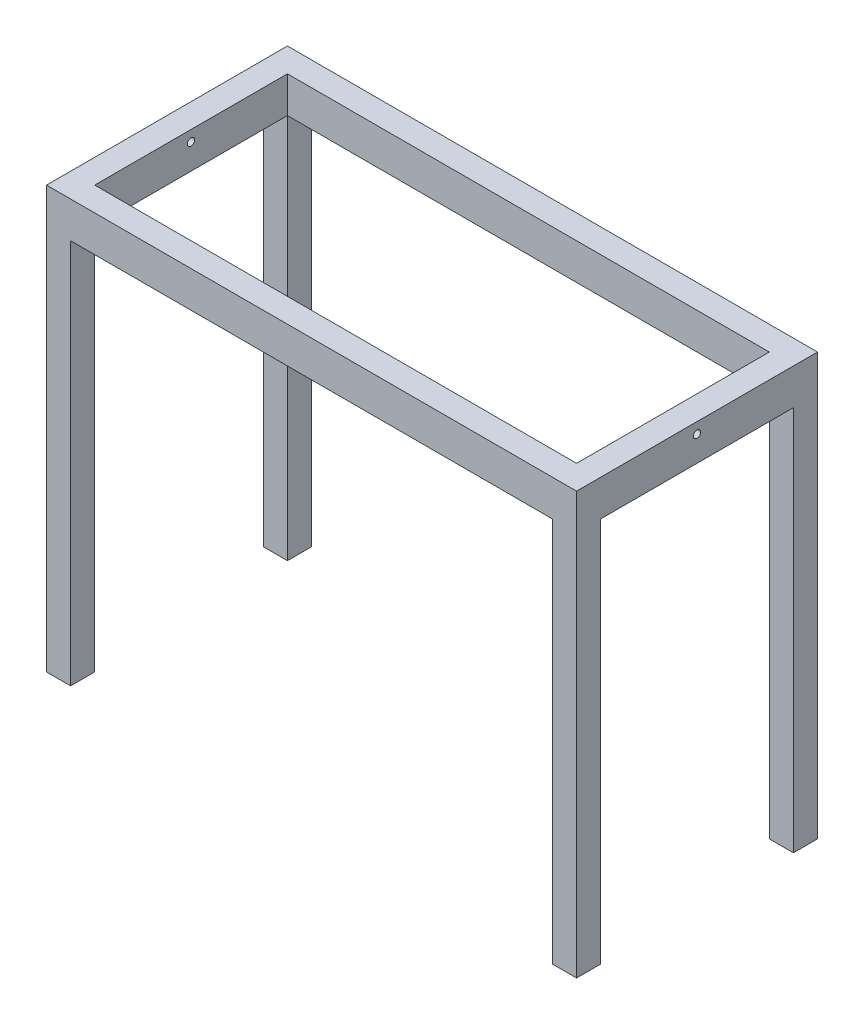
from build123d import *

# Parameters (mm, degrees)
SKETCH1_W               = 1100
SKETCH1_H               = 500
SKETCH1_W_2             = 1000
SKETCH1_H_2             = 400
BOSS_EXTRUDE1_DEPTH     = 75
SKETCH2_W               = 50
SKETCH2_H               = 50
BOSS_EXTRUDE2_DEPTH     = 800
CUT_EXTRUDE1_DEPTH      = 1383.931668594
CUT_EXTRUDE1_DEPTH_BACK = 1383.931668594
SKETCH3_R               = 7.5


with BuildPart() as part:
    # Sketch1 → Boss-Extrude1 (new body)
    with BuildSketch(Plane(origin=(0, 0, 0), x_dir=(1, 0, 0), z_dir=(0, 1, 0))):
        Rectangle(SKETCH1_W, SKETCH1_H)
        Rectangle(SKETCH1_W_2, SKETCH1_H_2, mode=Mode.SUBTRACT)
    extrude(amount=BOSS_EXTRUDE1_DEPTH)

    # Sketch2 → Boss-Extrude2 (add)
    with BuildSketch(Plane.XZ):
        with Locations((-525, 225)):
            Rectangle(SKETCH2_W, SKETCH2_H)
        with Locations((525, 225)):
            Rectangle(SKETCH2_W, SKETCH2_H)
        with Locations((525, -225)):
            Rectangle(SKETCH2_W, SKETCH2_H)
        with Locations((-525, -225)):
            Rectangle(SKETCH2_W, SKETCH2_H)
    extrude(amount=BOSS_EXTRUDE2_DEPTH)

    # Sketch3 → Cut-Extrude1 (cut, two sides: drawn at the far end of the back side and taken through both)
    with BuildSketch(Plane.ZY.offset(550).offset(-CUT_EXTRUDE1_DEPTH_BACK)):
        with Locations(Location((0, 52.5, 0), (0, 0, 180))):
            Circle(SKETCH3_R)
    extrude(amount=CUT_EXTRUDE1_DEPTH + CUT_EXTRUDE1_DEPTH_BACK, mode=Mode.SUBTRACT)


solid = part.part
